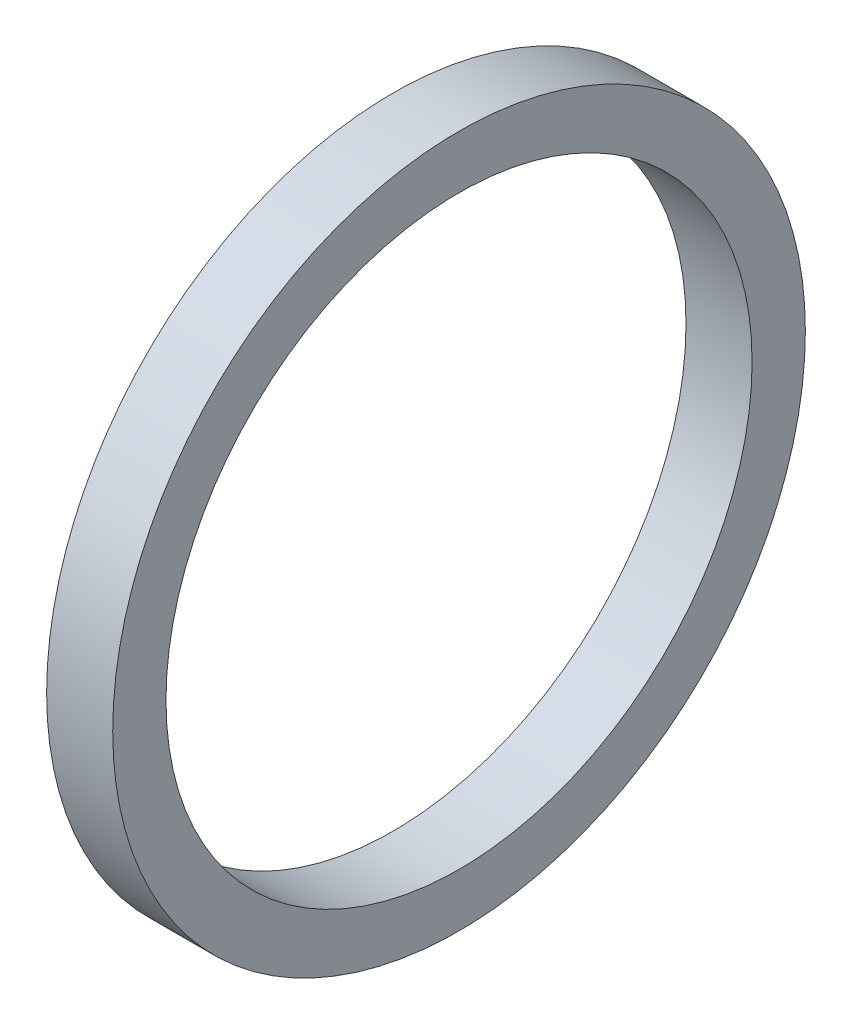
from build123d import *

# Parameters (mm, degrees)
SKETCH2_R           = 32.5
SKETCH2_R_2         = 27.5
BOSS_EXTRUDE1_DEPTH = 6.2


with BuildPart() as part:
    # Sketch2 → Boss-Extrude1 (new body)
    with BuildSketch(Plane(origin=(0, 0, 0), x_dir=(0, 0, -1), z_dir=(1, 0, 0))):
        with Locations(Location((0, 0, 0), (0, 0, 180))):
            Circle(SKETCH2_R)
        with Locations(Location((0, 0, 0), (0, 0, 180))):
            Circle(SKETCH2_R_2, mode=Mode.SUBTRACT)
    extrude(amount=BOSS_EXTRUDE1_DEPTH)


solid = part.part
